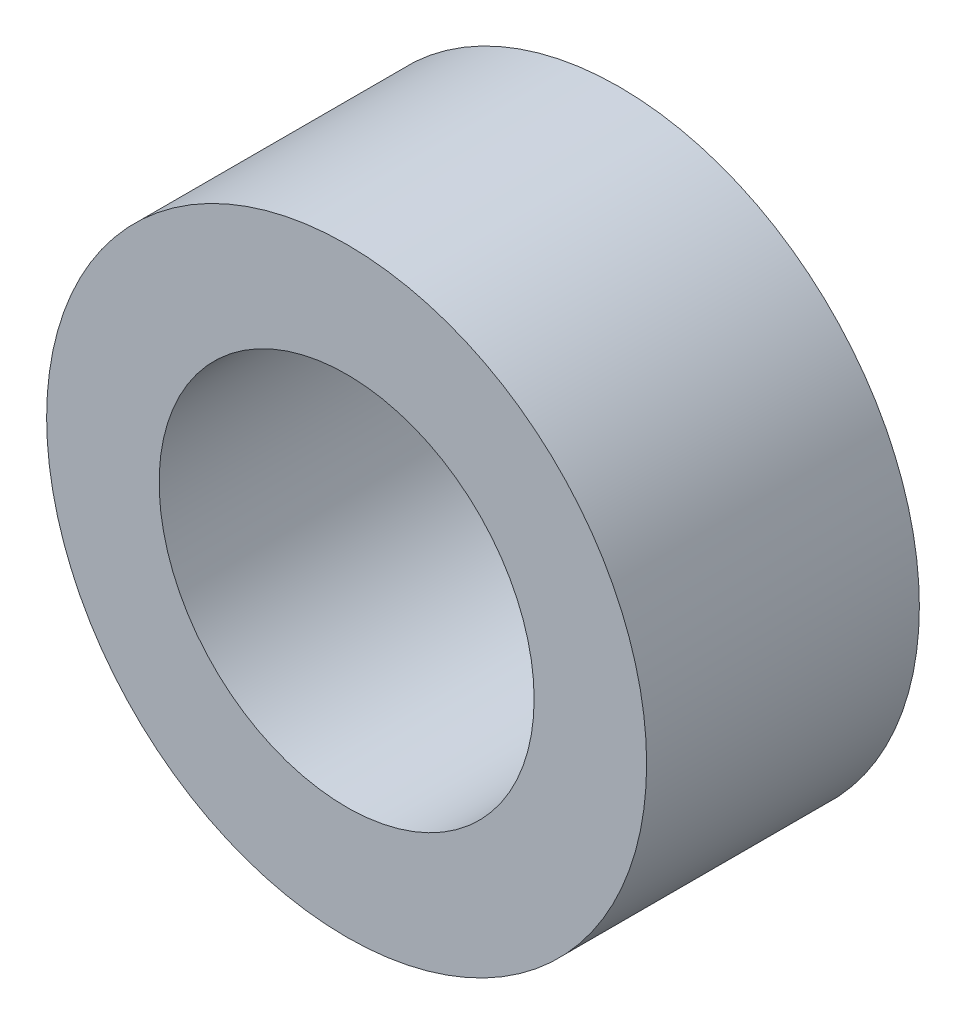
SolidWorks part; units mm, degrees
ref_plane "Front Plane" through (0, 0, 0) normal (0, 0, 1) x (1, 0, 0)
ref_plane "Top Plane" through (0, 0, 0) normal (0, 1, 0) x (1, 0, 0)
ref_plane "Right Plane" through (0, 0, 0) normal (1, 0, 0) x (0, 0, -1)
sketch "Sketch1" plane through (0, 0, 0) normal (0, 0, 1) x (1, 0, 0)
  circle A0 centre (0, 0) radius 4.4
  circle A1 centre (0, 0) radius 2.75
  dimension "D1" = 8.8
  dimension "D2" = 5.5
extrude "Boss-Extrude1" add sketch "Sketch1" along normal blind 4
